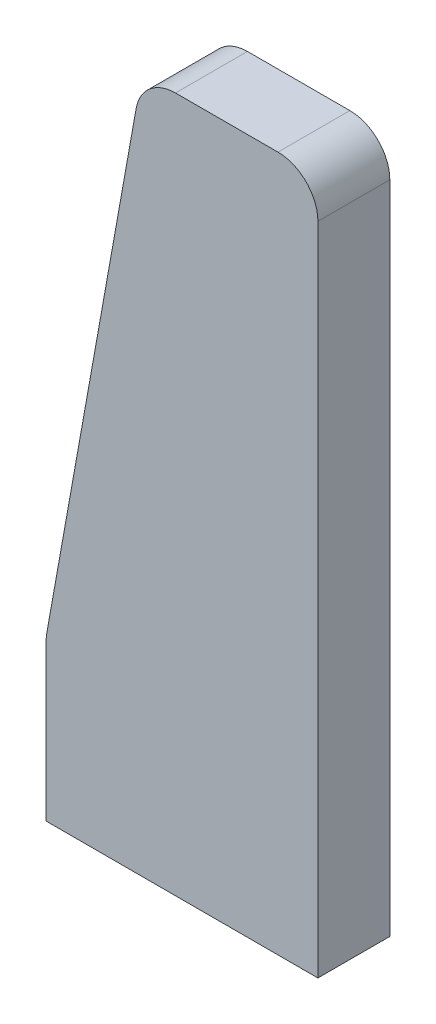
from build123d import *

# Parameters (mm, degrees)
BOSS_EXTRUDE1_DEPTH = 9


with BuildPart() as part:
    # Sketch1 → Boss-Extrude1 (new body)
    with BuildSketch(Plane.XY):
        with BuildLine():
            Line((0, 0), (-34, 0))
            Line((-34, 0), (-34, 19.555773208))
            ThreePointArc((-34, 19.555773208), (-33.980382319, 19.99825706), (-33.921683216, 20.437268709))
            Line((-33.921683216, 20.437268709), (-22.737642597, 82.881495501))
            ThreePointArc((-22.737642597, 82.881495501), (-21.024738159, 85.834545443), (-17.815959381, 87))
            Line((-17.815959381, 87), (-5, 87))
            ThreePointArc((-5, 87), (-1.464466094, 85.535533906), (0, 82))
            Line((0, 82), (0, 0))
        make_face()
    extrude(amount=BOSS_EXTRUDE1_DEPTH)


solid = part.part
